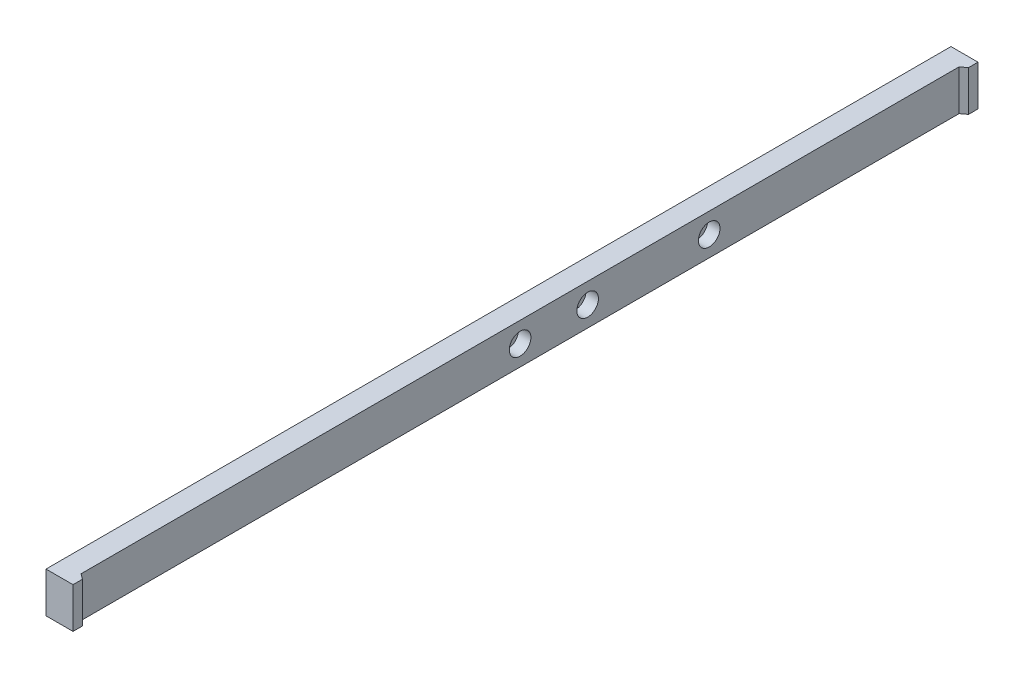
SolidWorks part; units mm, degrees
material "AL6061"
ref_plane "Front Plane" through (0, 0, 0) normal (0, 0, 1) x (1, 0, 0)
ref_plane "Top Plane" through (0, 0, 0) normal (0, 1, 0) x (1, 0, 0)
ref_plane "Right Plane" through (0, 0, 0) normal (1, 0, 0) x (0, 0, -1)
sketch "Sketch1" plane through (0, 0, 0) normal (1, 0, 0) x (0, 0, -1)
  line L1 (-167.5, -7.5) -> (167.5, -7.5)
  line L2 (-167.5, -7.5) -> (-167.5, 7.5)
  line L3 (-167.5, 7.5) -> (167.5, 7.5)
  line L4 (167.5, -7.5) -> (167.5, 7.5)
  line L5 (-167.5, -7.5) -> (167.5, 7.5) construction
  line L6 (-167.5, 7.5) -> (167.5, -7.5) construction
  point P0 (0, 0)
  dimension "D1" = 335
  dimension "D2" = 15
extrude "Boss-Extrude1" add sketch "Sketch1" along normal blind 10
sketch "Sketch2" plane through (0, -7.5, 0) normal (0, -1, 0) x (1, 0, 0)
  line L0 (0, 0) -> (10, 0) construction
  line L1 (10, 167.5) -> (10, -167.5) construction
  line L4 (8, 162.5) -> (8, -162.5)
  line L5 (10, 164) -> (8, 162.5)
  line L6 (10, -164) -> (8, -162.5)
  line L9 (10, 164) -> (10, 0)
  line L10 (10, 0) -> (10, -164)
  point P12 (8, 0)
  dimension "D1" = 2
  dimension "D2" = 325
  dimension "D3" = 1.5
extrude "Cut-Extrude2" cut sketch "Sketch2" against normal through all
hole_wizard "CBORE for M4 Hexagon socket head cap screws1" positions "Sketch3" profile "Sketch4" counterbore size "M4" standard "GB" end condition through all
sketch "Sketch3" plane through (8, 0, 0) normal (1, 0, 0) x (0, 0, -1)
  point P0 (0, 0)
  point P5 (70, 0)
  point P7 (25, 0)
  dimension "D1" = 45
  dimension "D2" = 70
sketch "Sketch4" plane through (8, 0, 0) normal (0, 1, 0) x (0, 0, -1)
  line L0 (0, 0) -> (0, 8)
  line L1 (0, 8) -> (2.25, 8)
  line L3 (2.25, 8) -> (2.25, 4.6)
  line L4 (2.25, 4.6) -> (4, 4.6)
  line L5 (4, 4.6) -> (4, 0)
  line L7 (4, 0) -> (0, 0)
  line L11 (0, -6.35) -> (0, 107.95) construction
  dimension "通孔孔直径" = 4.5
  dimension "通孔孔深度" = 8
  dimension "柱形沉头孔直径" = 8
  dimension "柱形沉头孔深度" = 4.6
